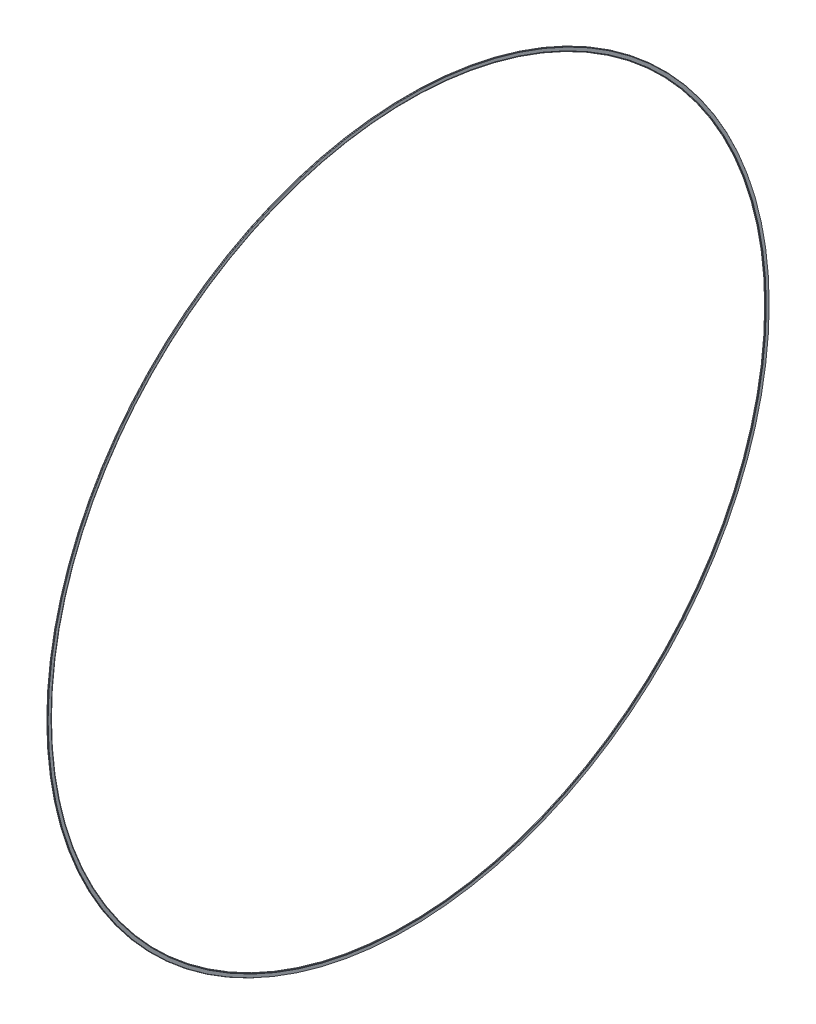
SolidWorks part; units mm, degrees
ref_plane "前视基准面" through (0, 0, 0) normal (0, 0, 1) x (1, 0, 0)
ref_plane "上视基准面" through (0, 0, 0) normal (0, 1, 0) x (1, 0, 0)
ref_plane "右视基准面" through (0, 0, 0) normal (1, 0, 0) x (0, 0, -1)
sketch "草图1" plane through (0, 0, 0) normal (0, 0, 1) x (1, 0, 0)
  line L0 (0, 0) -> (0, 148.3) construction
  line L1 (0, 148.3) -> (0.15, 148.3)
  line L2 (0.4, 148.158) -> (0.4, 146.936)
  line L3 (0.4, 146.936) -> (0.3121, 146.7)
  line L4 (0.3121, 146.7) -> (0, 146.7)
  line L5 (0, 146.7) -> (0, 148.3)
  line L6 (0, 0) -> (2.6472, 0) construction
  arc A0 (0.15, 148.3) -> (0.4, 148.158) centre (0.4406, 148.5206) ccw
  dimension "D4" = 0.3648
  dimension "D1" = 0.4
  dimension "D2" = 1.6
  dimension "D3" = 0.15
  dimension "D5" = 148.3
  dimension "D6" = 0.236
revolve "旋转1" add sketch "草图1" angle 360 about L6
